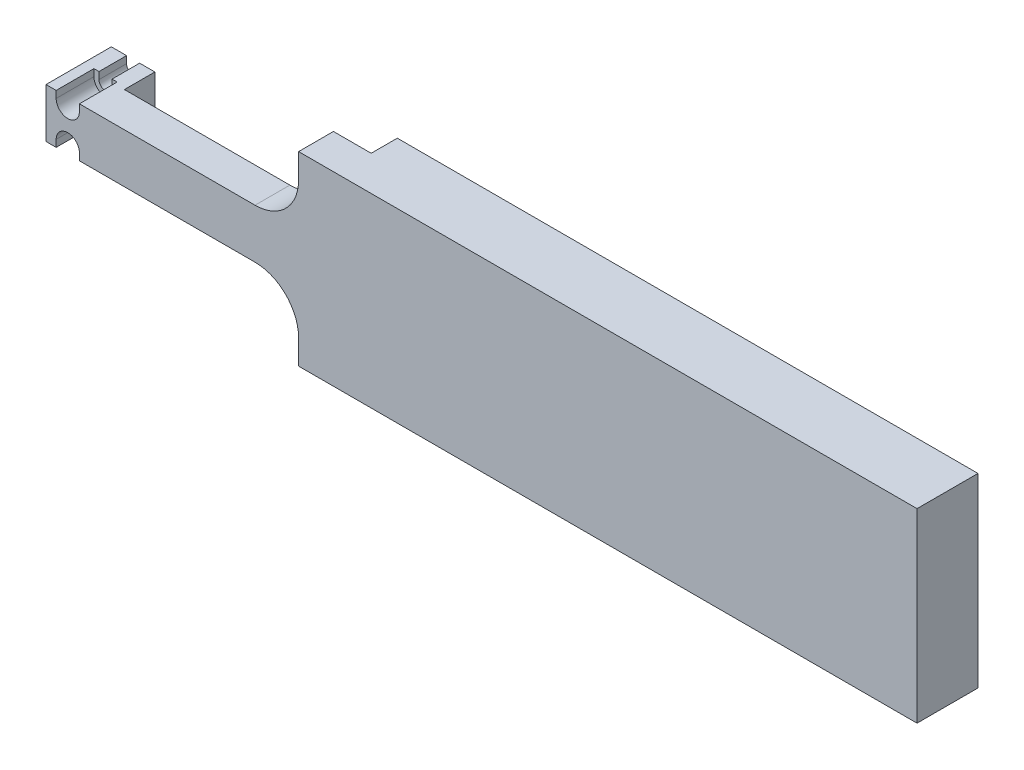
SolidWorks part; units mm, degrees
ref_plane "前视基准面" through (0, 0, 0) normal (0, 0, 1) x (1, 0, 0)
ref_plane "上视基准面" through (0, 0, 0) normal (0, 1, 0) x (1, 0, 0)
ref_plane "右视基准面" through (0, 0, 0) normal (1, 0, 0) x (0, 0, -1)
sketch "草图1" plane through (0, 0, 0) normal (0, 1, 0) x (1, 0, 0)
  line L0 (0, 0) -> (-200, 0)
  line L1 (-200, 0) -> (-200, -9)
  line L2 (-200, -9) -> (-285, -9)
  line L3 (-285, -9) -> (-285, 1.5)
  line L4 (-285, 1.5) -> (-300, 1.5)
  line L5 (-300, 1.5) -> (-300, -21)
  line L6 (-300, -21) -> (0, -21)
  line L7 (0, -21) -> (0, 0)
  dimension "D1" = 200
  dimension "D2" = 1.5
  dimension "D3" = 9
  dimension "D4" = 15
  dimension "D5" = 85
  dimension "D6" = 12
extrude "凸台-拉伸1" add sketch "草图1" along normal mid plane 64
sketch "草图2" plane through (0, 0, -1.5) normal (0, 0, -1) x (-1, 0, 0)
  line L1 (300, -32) -> (213, -32)
  line L2 (300, -32) -> (300, -8.5)
  line L3 (300, -8.5) -> (213, -8.5)
  line L4 (213, -32) -> (213, -8.5)
  line L5 (300, 32) -> (213, 32)
  line L6 (300, 32) -> (300, 8.5)
  line L7 (300, 8.5) -> (213, 8.5)
  line L8 (213, 32) -> (213, 8.5)
  point P10 (256.5, 8.5)
  dimension "D1" = 17
  dimension "D2" = 87
extrude "切除-拉伸1" cut sketch "草图2" against normal up to surface (22.5 mm away) up to face at (-150, 0, 21)
fillet "圆角1" radius 15 2 edges at (-213, 8.5, 15) (-213, -8.5, 15)
sketch "草图5" plane through (0, 0, 21) normal (0, 0, 1) x (1, 0, 0)
  line L0 (-300, 8.5) -> (-228, 8.5) construction
  line L1 (-296, -8.5) -> (-289, -8.5)
  line L2 (-296, -8.5) -> (-296, 8.5)
  line L3 (-296, 8.5) -> (-289, 8.5)
  line L4 (-289, -8.5) -> (-289, 8.5)
  line L5 (-296, -8.5) -> (-289, 8.5) construction
  line L6 (-296, 8.5) -> (-289, -8.5) construction
  line L7 (-300, 8.5) -> (-300, -8.5) construction
  line L8 (-228, -8.5) -> (-300, -8.5) construction
  point P0 (-292.5, 0)
  dimension "D1" = 7
  dimension "D2" = 7.5
sketch "草图7" plane through (0, 0, 21) normal (0, 0, 1) x (1, 0, 0)
  line L0 (-296.5, 8.5) -> (-296.5, 6.1)
  line L1 (-300, 8.5) -> (-228, 8.5) construction
  line L2 (-288.5, 6.1) -> (-288.5, 8.5)
  line L4 (-288.5, 8.5) -> (-296.5, 8.5)
  line L5 (-300, 8.5) -> (-300, -8.5) construction
  arc A0 (-296.5, 6.1) -> (-288.5, 6.1) centre (-292.5, 6.1) ccw
  dimension "D2" = 4
  dimension "D1" = 7.5
  dimension "D3" = 2.4
extrude "切除-拉伸2" cut sketch "草图7" against normal blind 13
sketch "草图8" plane through (0, 0, 8) normal (0, 0, 1) x (1, 0, 0)
  line L0 (-290.25, 6.1) -> (-290.25, 8.5)
  line L1 (-296, 8.5) -> (-289, 8.5) construction
  line L2 (-290.25, 8.5) -> (-294.75, 8.5)
  line L3 (-294.75, 8.5) -> (-294.75, 6.1)
  arc A0 (-294.75, 6.1) -> (-290.25, 6.1) centre (-292.5, 6.1) ccw
  dimension "D1" = 4.5
extrude "切除-拉伸3" cut sketch "草图8" against normal up to next
mirror "镜向1" about plane through (0, 0, 0) normal (0, 1, 0) of "切除-拉伸2", "切除-拉伸3"
sketch "草图9" plane through (0, 0, 21) normal (0, 0, 1) x (1, 0, 0)
  line L0 (0, 32) -> (0, -32) construction
  line L1 (-60, -25) -> (0, -25)
  line L2 (-60, -25) -> (-60, 25)
  line L3 (-60, 25) -> (0, 25)
  line L4 (0, -25) -> (0, 25)
  line L5 (-60, -25) -> (0, 25) construction
  line L6 (-60, 25) -> (0, -25) construction
  point P0 (-30, 0)
  dimension "D1" = 50
  dimension "D2" = 60
extrude "切除-拉伸4" [suppressed] cut sketch "草图9" against normal blind 2
fillet "圆角3" [suppressed] radius 5
